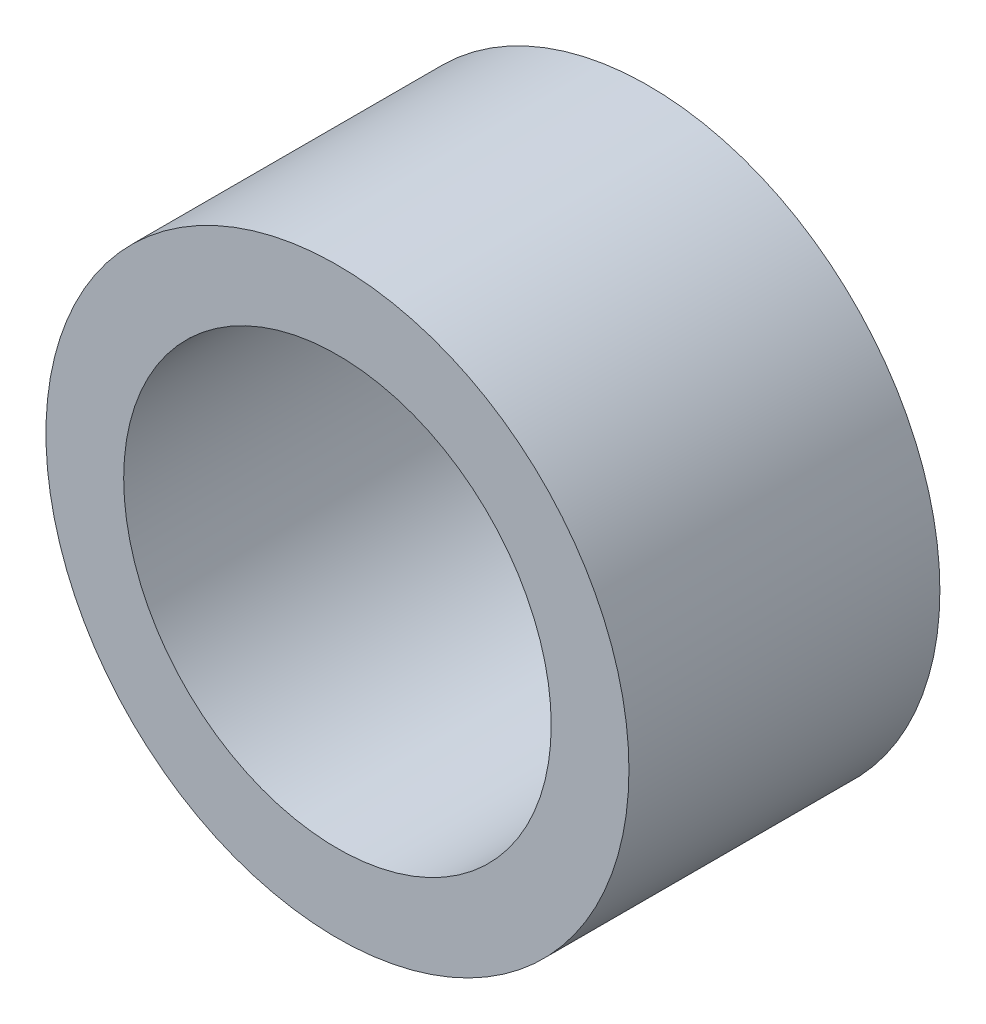
from build123d import *

# Parameters (mm, degrees)
SKETCH_1_R      = 7.5
SKETCH_1_R_2    = 5.5
EXTRUDE_1_DEPTH = 8


with BuildPart() as part:
    # 草图1 → 凸台-拉伸1 (new body)
    with BuildSketch(Plane.XY):
        Circle(SKETCH_1_R)
        Circle(SKETCH_1_R_2, mode=Mode.SUBTRACT)
    extrude(amount=EXTRUDE_1_DEPTH)


solid = part.part
